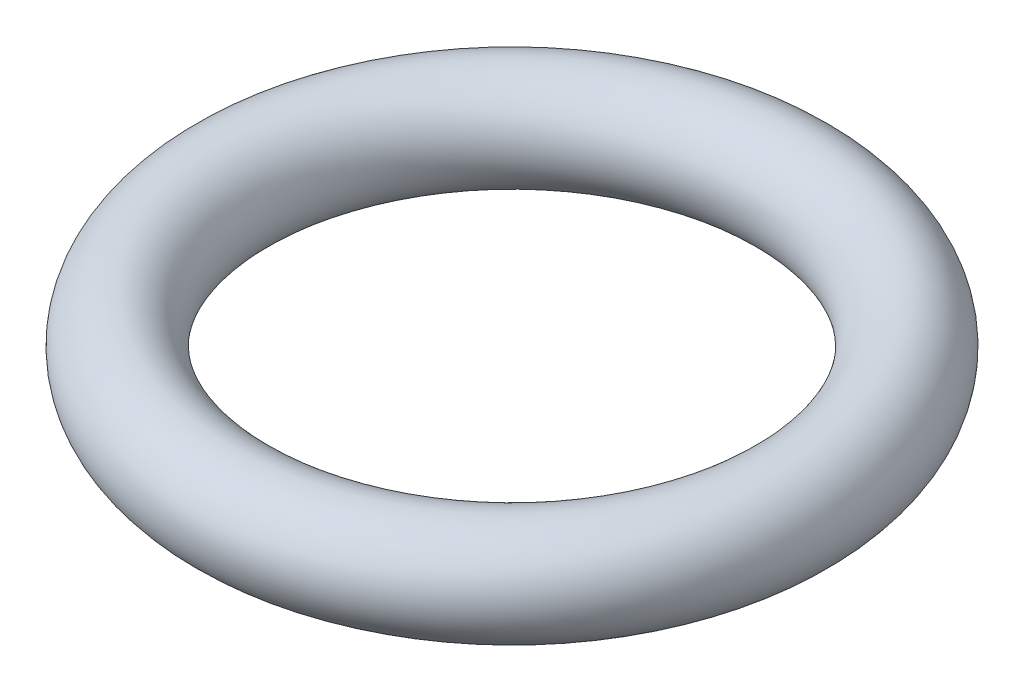
SolidWorks part; units mm, degrees
ref_plane "Front Plane" through (0, 0, 0) normal (0, 0, 1) x (1, 0, 0)
ref_plane "Top Plane" through (0, 0, 0) normal (0, 1, 0) x (1, 0, 0)
ref_plane "Right Plane" through (0, 0, 0) normal (1, 0, 0) x (0, 0, -1)
other "Configuration Table"
sketch "Sketch1" plane through (0, 0, 0) normal (0, 1, 0) x (1, 0, 0)
  circle A0 centre (0, 0) radius 5.1016 construction
  circle A1 centre (0, 0) radius 5.1016
sweep "Sweep1" add path "Sketch1" circular profile diameter 1.84 parameters "D3"=1.84
ref_plane "Plane1" through (0, 0.92, 0) normal (0, 1, 0) x (1, 0, 0)
sketch "Sketch5" plane through (0, 0.92, 0) normal (0, 1, 0) x (1, 0, 0)
  circle A0 centre (0, 0) radius 5.1016 construction
  circle A1 centre (0, 0) radius 5.1016
